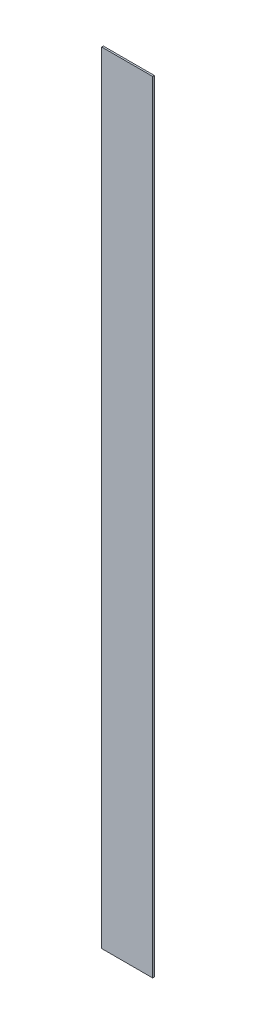
SolidWorks part; units mm, degrees
material "PMMA(有机玻璃)"
ref_plane "前视" through (0, 0, 0) normal (0, 0, 1) x (1, 0, 0)
ref_plane "上视" through (0, 0, 0) normal (0, 1, 0) x (1, 0, 0)
ref_plane "右视" through (0, 0, 0) normal (1, 0, 0) x (0, 0, -1)
sketch "草图1" plane through (0, 0, 0) normal (0, 0, 1) x (1, 0, 0)
  line L1 (-75.5, 1155) -> (75.5, 1155)
  line L2 (-75.5, 1155) -> (-75.5, -1155)
  line L3 (-75.5, -1155) -> (75.5, -1155)
  line L4 (75.5, 1155) -> (75.5, -1155)
  line L5 (-75.5, 1155) -> (75.5, -1155) construction
  line L6 (-75.5, -1155) -> (75.5, 1155) construction
  point P0 (0, 0)
  dimension "D1" = 2310
  dimension "D2" = 151
extrude "凸台-拉伸1" add sketch "草图1" along normal blind 5
hole_wizard "M5 间隙孔1" positions "草图3" profile "草图2" hole size "M5" standard "GB"
sketch "草图3" plane through (0, 0, 5) normal (0, 0, 1) x (1, 0, 0)
  line L0 (-427.5, 273) -> (-427.5, -273) construction
  line L1 (-427.5, -273) -> (427.5, -273) construction
  line L2 (0, 273) -> (0, -273) construction
  line L3 (427.5, 273) -> (-427.5, 273) construction
  line L5 (-427.5, 0) -> (427.5, 0) construction
  line L6 (427.5, -273) -> (427.5, 273) construction
  point P0 (-375, -261)
  point P46 (415.5, 250)
  point P48 (-415.5, 250)
  point P58 (-125, -261)
  point P59 (125, -261)
  point P61 (-125, 261)
  point P62 (125, 261)
  point P64 (-375, 261)
  point P88 (375, -261)
  point P89 (375, 261)
  point P108 (415.5, 0)
  point P109 (-415.5, 0)
  point P110 (415.5, -250)
  point P111 (-415.5, -250)
  dimension "D1" = 12
  dimension "D2" = 12
  dimension "D5" = 3
  dimension "D3" = 12
  dimension "D6" = 4
  dimension "D4" = 2
sketch "草图2" plane through (-375, -261, 5) normal (1, 0, 0) x (0, -1, 0)
  line L0 (0, 0) -> (0, 5)
  line L1 (0, 5) -> (2.75, 5)
  line L2 (2.75, 5) -> (2.75, 0)
  line L5 (2.75, 0) -> (0, 0)
  line L11 (0, -6.35) -> (0, 107.95) construction
  dimension "通孔孔直径" = 5.5
  dimension "通孔孔深度" = 5
